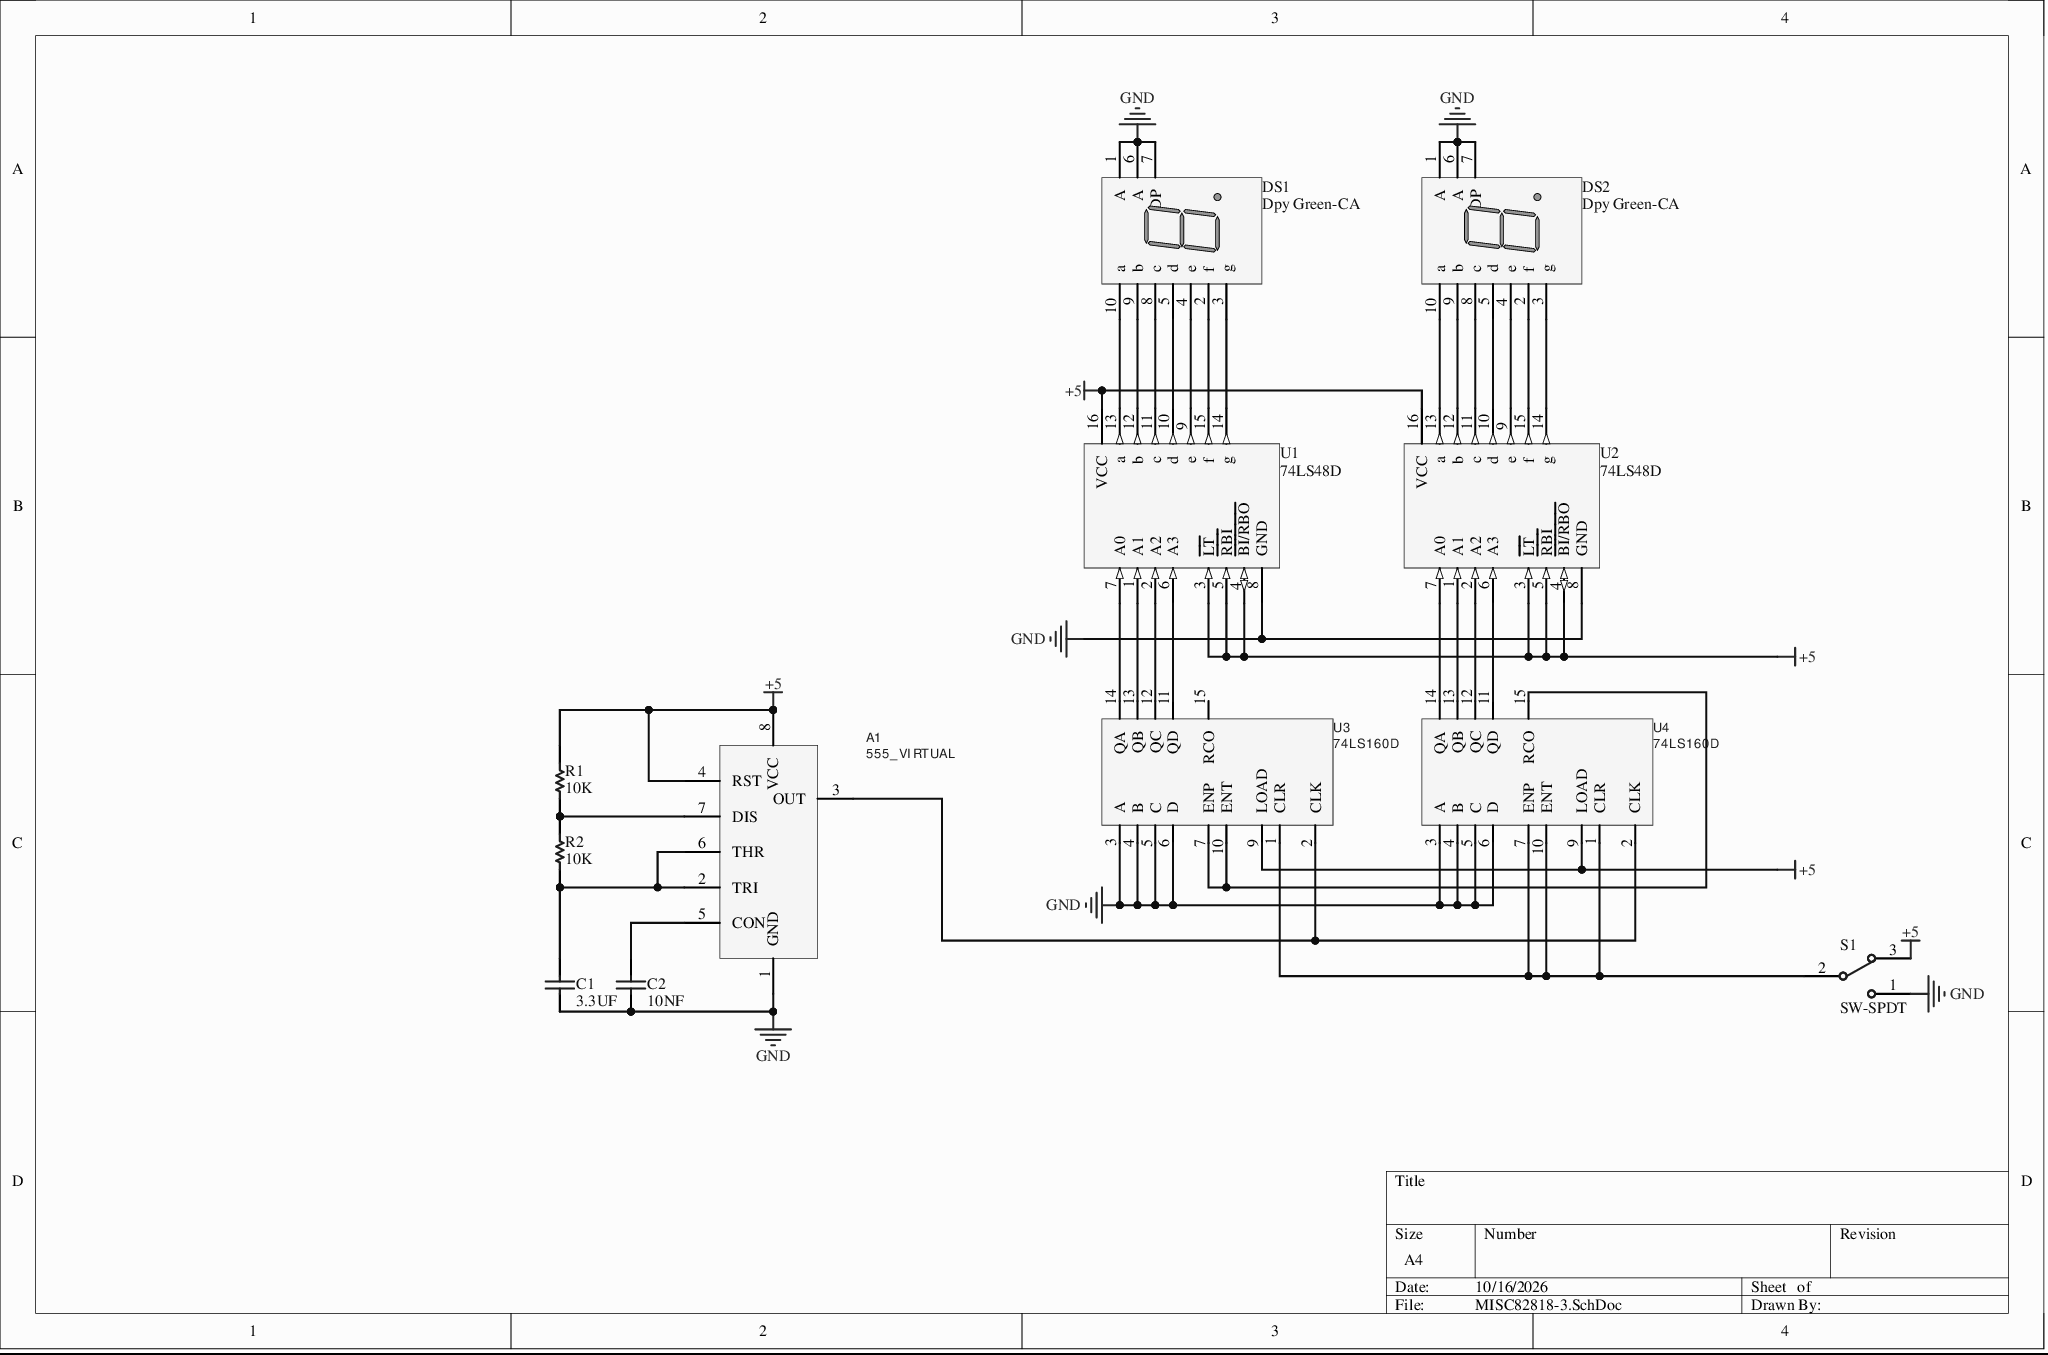
[diagram p0: MISC82818-3.SchDoc]
# Altium project MISC82818-2.PrjPcb
1 sheet, 12 parts. Net scope: global (net labels, ports and power ports of the same name join across sheets).
Board file: MISC82818.PcbDoc

## Sheet MISC82818-3.SchDoc
size A4

### Parts
A1  555_VIRTUAL  [DIP8]
C1  3.3UF  [RAD-0.3]
C2  10NF  [RAD-0.3]
DS1  Dpy Green-CA  [A]
DS2  Dpy Green-CA  [A]
R1  10K  [AXIAL-0.3]
R2  10K  [AXIAL-0.3]
S1  SW-SPDT  [SW-SPDT-3]
U1  74LS48D  [DIP16]
U2  74LS48D  [DIP16]
U3  74LS160D  [DIP16]
U4  74LS160D  [DIP16]

### Nets
+5: A1.4(RST) A1.8(VCC) R1.2 S1.3 U1.3(~{LT}) U1.4(~{BI/RBO}) U1.5(~{RBI}) U1.16(VCC) U2.3(~{LT}) U2.4(~{BI/RBO}) U2.5(~{RBI}) U2.16(VCC) U3.9(LOAD) U4.9(LOAD)
GND: A1.1(GND) C1.1 C2.1 DS1.1(A) DS1.6(A) DS1.7(DP) DS2.1(A) DS2.6(A) DS2.7(DP) S1.1 U1.8(GND) U2.8(GND) U3.3(A) U3.4(B) U3.5(C) U3.6(D) U4.3(A) U4.4(B) U4.5(C) U4.6(D)
NetA1_2: A1.2(TRI) A1.6(THR) C1.2 R2.1
NetA1_3: A1.3(OUT) U3.2(CLK) U4.2(CLK)
NetA1_5: A1.5(CON) C2.2
NetA1_7: A1.7(DIS) R1.1 R2.2
NetDS1_2: DS1.2(f) U1.15(f)
NetDS1_3: DS1.3(g) U1.14(g)
NetDS1_4: DS1.4(e) U1.9(e)
NetDS1_5: DS1.5(d) U1.10(d)
NetDS1_8: DS1.8(c) U1.11(c)
NetDS1_9: DS1.9(b) U1.12(b)
NetDS1_10: DS1.10(a) U1.13(a)
NetDS2_2: DS2.2(f) U2.15(f)
NetDS2_3: DS2.3(g) U2.14(g)
NetDS2_4: DS2.4(e) U2.9(e)
NetDS2_5: DS2.5(d) U2.10(d)
NetDS2_8: DS2.8(c) U2.11(c)
NetDS2_9: DS2.9(b) U2.12(b)
NetDS2_10: DS2.10(a) U2.13(a)
NetS1_2: S1.2 U3.1(CLR) U4.1(CLR) U4.7(ENP) U4.10(ENT)
NetU1_1: U1.1(A1) U3.13(QB)
NetU1_2: U1.2(A2) U3.12(QC)
NetU1_6: U1.6(A3) U3.11(QD)
NetU1_7: U1.7(A0) U3.14(QA)
NetU2_1: U2.1(A1) U4.13(QB)
NetU2_2: U2.2(A2) U4.12(QC)
NetU2_6: U2.6(A3) U4.11(QD)
NetU2_7: U2.7(A0) U4.14(QA)
NetU3_7: U3.7(ENP) U3.10(ENT) U4.15(RCO)

Not connected (* = marked no-connect by the designer): U3 15(RCO)

### Library data of the parts
C1 C2 = Cap: Capacitor; Value: 100pF; Published: 8-Jun-2000; LatestRevisionDate: 17-Jul-2002; LatestRevisionNote: Re-released for DXP Platform.; PackageReference: RAD-0.3; PackageDescription: Radial Cap, Thru-Hole; 2 Leads; 0.3 in Pin Spacing; Publisher: Altium Limited
DS1 DS2 = Dpy Green-CA: 7.62 mm Black Surface Green 7-Segment Display: CA, RH DP; MinimumIntensity: 860 ucd; Note: IF = 10 mA; Note: Pins 1 and 6 are redundant Anodes.; Published: 8-Jun-2000; LatestRevisionDate: 17-Dec-2003; LatestRevisionNote: Schematic revised, PCB Footprint replaced.; DatasheetVersion: 19-Feb-2002; PackageVersion: 11-Feb-2002; PackageReference: A; PackageDescription: LED, 7-Segment Display, 7.62 mm, RHD; 10 Leads; Row Space 5.08 mm; Pitch 2.54 mm; Colour: Green; ComponentLink1Description: Manufacturer Link; ComponentLink1URL: http://www.agilent.com/; Publisher: Altium Limited
R1 R2 = Res1: Resistor; Value: 1K; Published: 8-Jun-2000; LatestRevisionDate: 17-Jul-2002; LatestRevisionNote: Re-released for DXP Platform.; PackageReference: AXIAL-0.3; PackageDescription: Axial Device, Thru-Hole; 2 Leads; 0.3 in Pin Spacing; Publisher: Altium Limited
S1 = SW-SPDT: SPDT Subminiature Toggle Switch, Right Angle Mounting, Vertical Actuation; Published: 24-Mar-1999; LatestRevisionDate: 17-Dec-2003; LatestRevisionNote: Schematic revised, PCB Footprint replaced.; DatasheetVersion: 05-Dec-2000; PackageReference: TL36WW15050; PackageDescription: Switch; 4 Leads; ComponentLink1Description: Manufacturer Link; ComponentLink1URL: http://www.apem.com; Publisher: Altium Limited
U1 U2 = SN74LS48D: BCD-to-Seven-Segment Decoder/Driver; Revision 1: 12-Jul-2000: SIM Model Added.; Revision 2: 17-Jul-2002: Re-released for DXP Platform.; Package Information: Latest Revision: Jan-1998; Published: 8-Jun-2000; Datasheet: 1988 TTL Logic Data Book (Mar-1988); Package Reference: D016; Publisher: Altium Limited